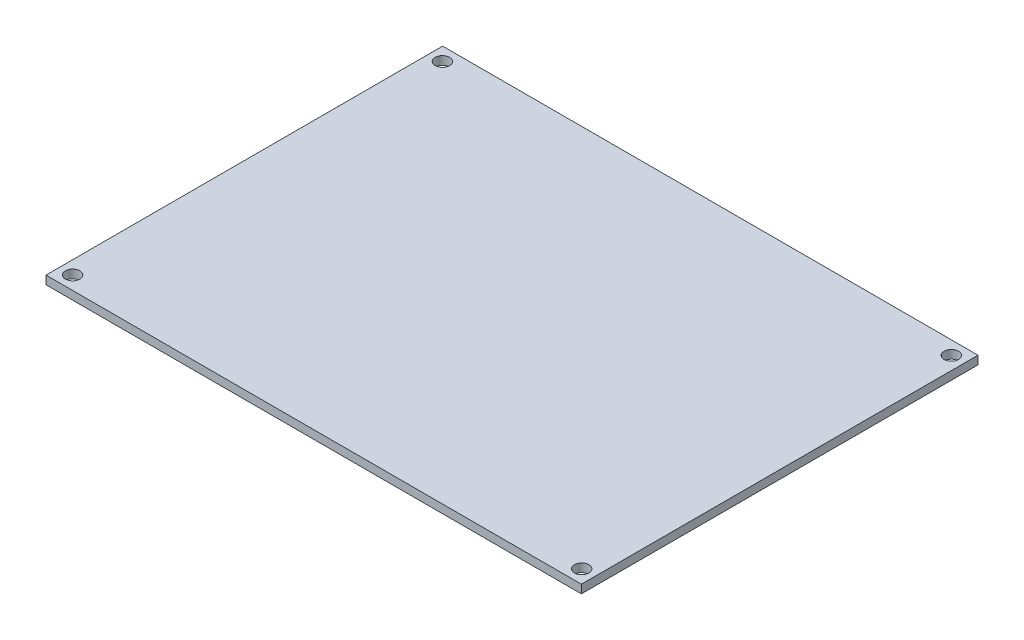
SolidWorks part; units mm, degrees
ref_plane "前视基准面" through (0, 0, 0) normal (0, 0, 1) x (1, 0, 0)
ref_plane "上视基准面" through (0, 0, 0) normal (0, 1, 0) x (1, 0, 0)
ref_plane "右视基准面" through (0, 0, 0) normal (1, 0, 0) x (0, 0, -1)
sketch "草图1" plane through (0, 0, 0) normal (0, 1, 0) x (1, 0, 0)
  line L0 (0, 41.3) -> (0, -41.3) construction
  line L1 (-55.75, -41.3) -> (55.75, -41.3)
  line L2 (-55.75, -41.3) -> (-55.75, 41.3)
  line L3 (-55.75, 41.3) -> (55.75, 41.3)
  line L4 (55.75, -41.3) -> (55.75, 41.3)
  line L5 (-55.75, -41.3) -> (55.75, 41.3) construction
  line L6 (-55.75, 41.3) -> (55.75, -41.3) construction
  line L7 (-55.75, 0) -> (55.75, 0) construction
  circle A0 centre (-53, 38.5) radius 1.5
  circle A1 centre (53, 38.5) radius 1.5
  circle A2 centre (53, -38.5) radius 1.5
  circle A3 centre (-53, -38.5) radius 1.5
  point P0 (0, 0)
  dimension "D1" = 106
  dimension "D4" = 3
  dimension "D5" = 1.3
  dimension "D2" = 111.5
  dimension "D3" = 82.6
extrude "凸台-拉伸1" add sketch "草图1" along normal blind 1.75
